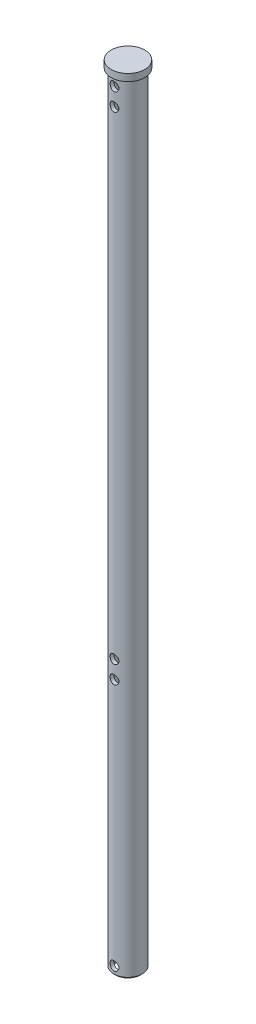
from build123d import *

# Parameters (mm, degrees)
SKETCH_1_R               = 19
EXTRUDE_1_DEPTH          = 8
SKETCH_2_R               = 16
SKETCH_2_R_2             = 12
EXTRUDE_2_DEPTH          = 880
CHAMFER_1_SIZE           = 2
CUT_EXTRUDE_2_DEPTH      = 881.4101317
CUT_EXTRUDE_2_DEPTH_BACK = 881.4101317
SKETCH_10_R              = 5


with BuildPart() as part:
    # 草图1 → 凸台-拉伸1 (new body)
    with BuildSketch(Plane(origin=(0, 0, 0), x_dir=(1, 0, 0), z_dir=(0, 1, 0))):
        with Locations(Location((0, 0, 0), (0, 0, 270))):
            Circle(SKETCH_1_R)
    extrude(amount=EXTRUDE_1_DEPTH)

    # 草图2 → 凸台-拉伸2 (add)
    with BuildSketch(Plane.XZ):
        with Locations(Location((0, 0, 0), (0, 0, 90))):
            Circle(SKETCH_2_R)
        with Locations(Location((0, 0, 0), (0, 0, 270))):
            Circle(SKETCH_2_R_2, mode=Mode.SUBTRACT)
    extrude(amount=EXTRUDE_2_DEPTH)

    # 倒角1
    chamfer_1_edges = [part.edges().sort_by_distance(p)[0] for p in [
        (0, -880, -16),
    ]]
    chamfer(chamfer_1_edges, length=CHAMFER_1_SIZE)

    # 草图10 → 切除-拉伸2 (cut, two sides: drawn at the far end of the back side and taken through both)
    with BuildSketch(Plane.XY.offset(-CUT_EXTRUDE_2_DEPTH_BACK)):
        with Locations((0, -870)):
            Circle(SKETCH_10_R)
        with Locations((0, -590)):
            Circle(SKETCH_10_R)
        with Locations((0, -570)):
            Circle(SKETCH_10_R)
        with Locations((0, -30)):
            Circle(SKETCH_10_R)
        with Locations((0, -10)):
            Circle(SKETCH_10_R)
    extrude(amount=CUT_EXTRUDE_2_DEPTH + CUT_EXTRUDE_2_DEPTH_BACK, mode=Mode.SUBTRACT)


solid = part.part
